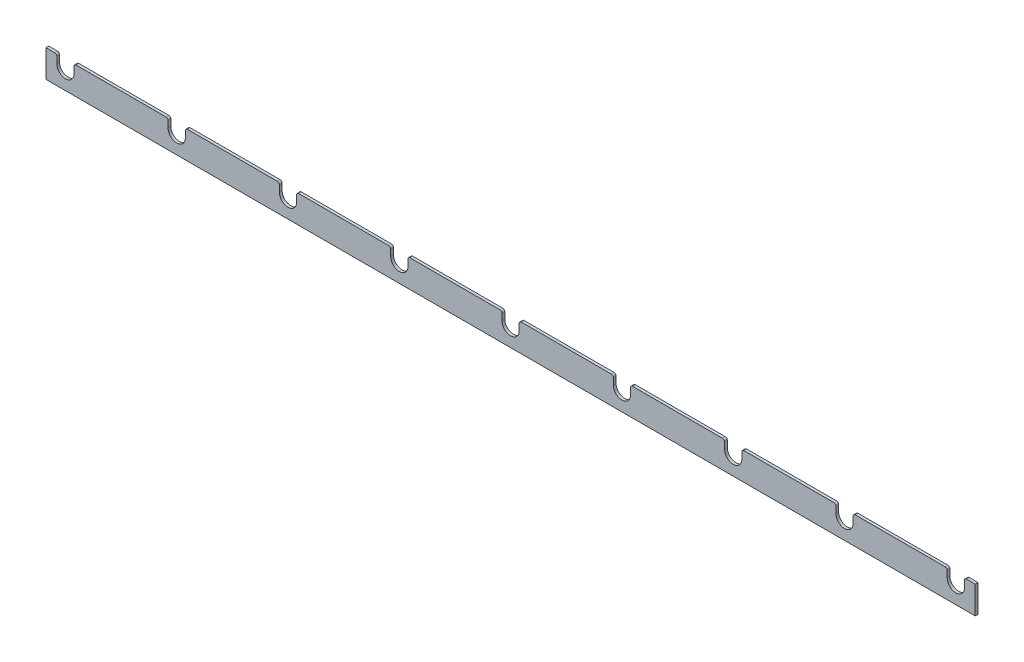
from build123d import *

# Parameters (mm, degrees)
SKETCH1_W           = 1350
SKETCH1_H           = 40
BOSS_EXTRUDE1_DEPTH = 4
CUT_EXTRUDE1_DEPTH  = 4
FILLET1_R           = 3


with BuildPart() as part:
    # Sketch1 → Boss-Extrude1 (new body)
    with BuildSketch(Plane.XY):
        Rectangle(SKETCH1_W, SKETCH1_H)
    extrude(amount=BOSS_EXTRUDE1_DEPTH)

    # Sketch2 → Cut-Extrude1 (cut)
    with BuildSketch(Plane.XY.offset(4)):
        with BuildLine():
            Line((-659.3, 7.5), (-659.3, 20))
            Line((-659.3, 20), (-634.3, 20))
            Line((-634.3, 20), (-634.3, 7.5))
            ThreePointArc((-634.3, 7.5), (-646.8, -5), (-659.3, 7.5))
        make_face()
        with BuildLine():
            Line((-497.6, 7.5), (-497.6, 20))
            Line((-497.6, 20), (-472.6, 20))
            Line((-472.6, 20), (-472.6, 7.5))
            ThreePointArc((-472.6, 7.5), (-485.1, -5), (-497.6, 7.5))
        make_face()
        with BuildLine():
            Line((-335.9, 7.5), (-335.9, 20))
            Line((-335.9, 20), (-310.9, 20))
            Line((-310.9, 20), (-310.9, 7.5))
            ThreePointArc((-310.9, 7.5), (-323.4, -5), (-335.9, 7.5))
        make_face()
        with BuildLine():
            Line((-174.2, 7.5), (-174.2, 20))
            Line((-174.2, 20), (-149.2, 20))
            Line((-149.2, 20), (-149.2, 7.5))
            ThreePointArc((-149.2, 7.5), (-161.7, -5), (-174.2, 7.5))
        make_face()
        with BuildLine():
            Line((-12.5, 7.5), (-12.5, 20))
            Line((-12.5, 20), (12.5, 20))
            Line((12.5, 20), (12.5, 7.5))
            ThreePointArc((12.5, 7.5), (0, -5), (-12.5, 7.5))
        make_face()
        with BuildLine():
            Line((149.2, 7.5), (149.2, 20))
            Line((149.2, 20), (174.2, 20))
            Line((174.2, 20), (174.2, 7.5))
            ThreePointArc((174.2, 7.5), (161.7, -5), (149.2, 7.5))
        make_face()
        with BuildLine():
            Line((310.9, 7.5), (310.9, 20))
            Line((310.9, 20), (335.9, 20))
            Line((335.9, 20), (335.9, 7.5))
            ThreePointArc((335.9, 7.5), (323.4, -5), (310.9, 7.5))
        make_face()
        with BuildLine():
            Line((472.6, 7.5), (472.6, 20))
            Line((472.6, 20), (497.6, 20))
            Line((497.6, 20), (497.6, 7.5))
            ThreePointArc((497.6, 7.5), (485.1, -5), (472.6, 7.5))
        make_face()
        with BuildLine():
            Line((634.3, 7.5), (634.3, 20))
            Line((634.3, 20), (659.3, 20))
            Line((659.3, 20), (659.3, 7.5))
            ThreePointArc((659.3, 7.5), (646.8, -5), (634.3, 7.5))
        make_face()
    extrude(amount=-CUT_EXTRUDE1_DEPTH, mode=Mode.SUBTRACT)

    # Fillet1
    fillet1_edges = [part.edges().sort_by_distance(p)[0] for p in [
        (497.6, 20, 2),
        (634.3, 20, 2),
        (659.3, 20, 2),
        (-659.3, 20, 2),
        (-634.3, 20, 2),
        (-497.6, 20, 2),
        (-472.6, 20, 2),
        (-335.9, 20, 2),
        (-310.9, 20, 2),
        (-174.2, 20, 2),
        (-149.2, 20, 2),
        (-12.5, 20, 2),
        (12.5, 20, 2),
        (149.2, 20, 2),
        (174.2, 20, 2),
        (310.9, 20, 2),
        (335.9, 20, 2),
        (472.6, 20, 2),
    ]]
    fillet(fillet1_edges, radius=FILLET1_R)


solid = part.part
